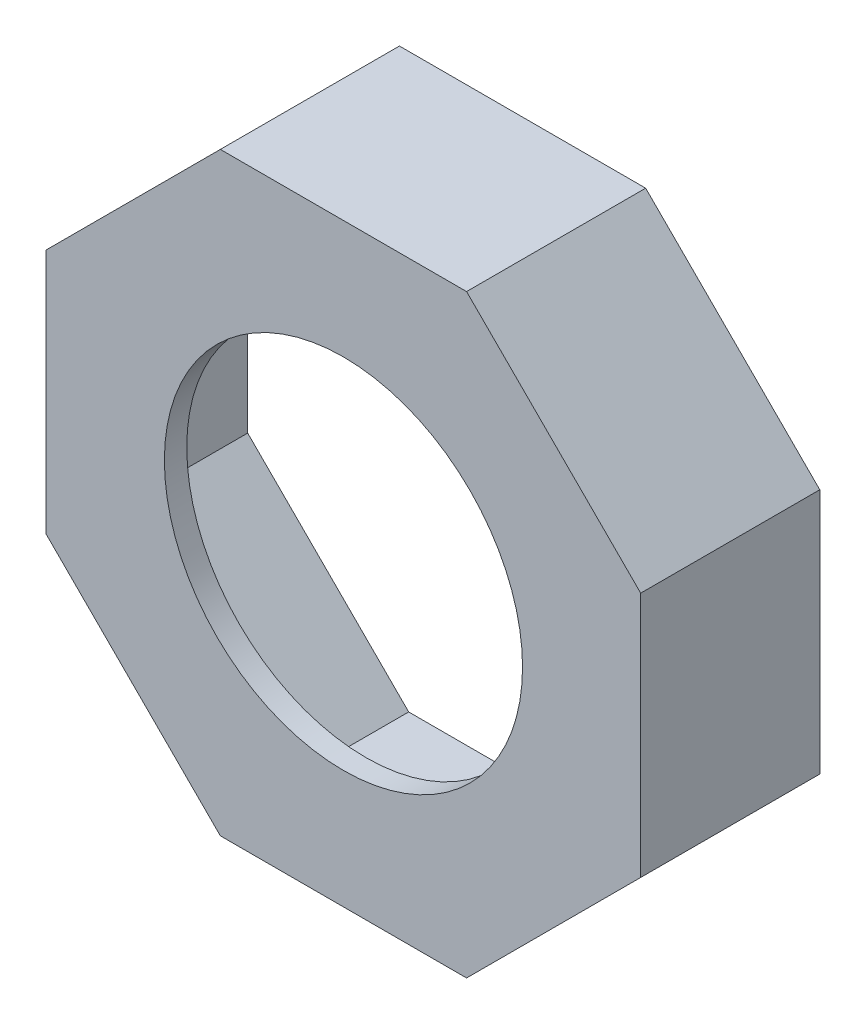
SolidWorks part; units mm, degrees
ref_plane "Front Plane" through (0, 0, 0) normal (0, 0, 1) x (1, 0, 0)
ref_plane "Top Plane" through (0, 0, 0) normal (0, 1, 0) x (1, 0, 0)
ref_plane "Right Plane" through (0, 0, 0) normal (1, 0, 0) x (0, 0, -1)
other "Configuration Table"
sketch "Sketch1" plane through (0, 0, 0) normal (0, 0, 1) x (1, 0, 0)
  line L1 (-467.1025, -35) -> (-544.8842, 42.7817)
  line L2 (-544.8842, 42.7817) -> (-654.8842, 42.7817)
  line L3 (-654.8842, 42.7817) -> (-732.6659, -35)
  line L4 (-732.6659, -35) -> (-732.6659, -145)
  line L5 (-732.6659, -145) -> (-654.8842, -222.7817)
  line L6 (-654.8842, -222.7817) -> (-544.8842, -222.7817)
  line L7 (-544.8842, -222.7817) -> (-467.1025, -145)
  line L8 (-467.1025, -145) -> (-467.1025, -35)
  circle A0 centre (-599.8842, -90) radius 132.7817 construction
  dimension "D1" = 110
extrude "Boss-Extrude1" add sketch "Sketch1" along normal blind 80
shell "Shell1" thickness 10
sketch "Sketch2" plane through (0, 0, 80) normal (0, 0, 1) x (1, 0, 0)
  circle A0 centre (-599.8842, -90) radius 80
  dimension "D1" = 160
extrude "Cut-Extrude1" cut sketch "Sketch2" against normal blind 80
